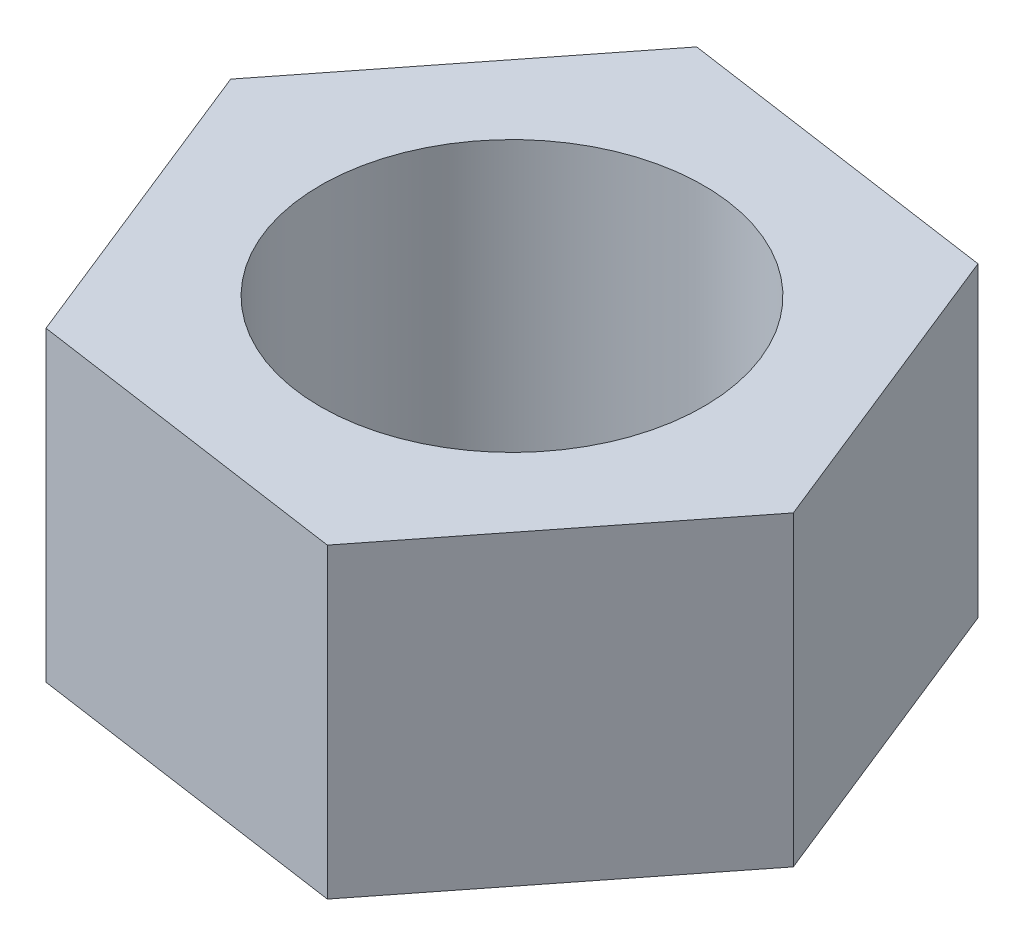
from build123d import *

# Parameters (mm, degrees)
SKETCH1_R           = 2
BOSS_EXTRUDE1_DEPTH = 3.2


with BuildPart() as part:
    # Sketch1 → Boss-Extrude1 (new body)
    with BuildSketch(Plane(origin=(0, 0, 0), x_dir=(1, 0, 0), z_dir=(0, 1, 0))):
        Polygon((2.14089179, 2.723340292), (-1.288035981, 3.215736823), (-3.428927771, 0.492396531), (-2.14089179, -2.723340292), (1.288035981, -3.215736823), (3.428927771, -0.492396531), align=None)
        with Locations(Location((0, 0, 0), (0, 0, 270))):
            Circle(SKETCH1_R, mode=Mode.SUBTRACT)
    extrude(amount=BOSS_EXTRUDE1_DEPTH)


solid = part.part
